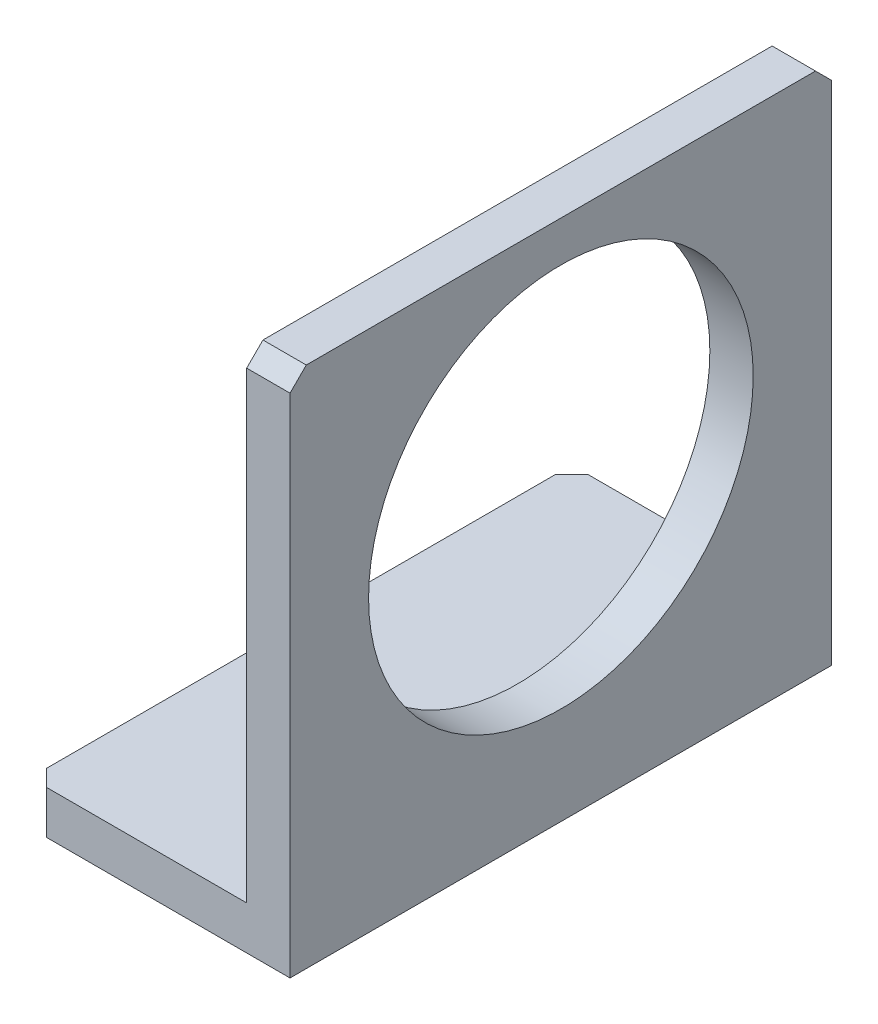
from build123d import *

# Parameters (mm, degrees)
EXTRUDE_1_DEPTH     = 50
CHAMFER_1_SIZE      = 3
CUT_EXTRUDE_1_REACH = 136.284
SKETCH_4_R          = 35.5


with BuildPart() as part:
    # 草图2 → 凸台-拉伸1 (new, symmetric)
    with BuildSketch(Plane(origin=(409.637600706, 0.5, -34.379468655), x_dir=(1, 0, 0), z_dir=(0, 0, 1))):
        Polygon((-409.637600706, 96), (-409.637600706, -0.5), (-457.637600706, -0.5), (-457.637600706, 7.5), (-417.637600706, 7.5), (-417.637600706, 96), align=None)
    extrude(amount=EXTRUDE_1_DEPTH, both=True)

    # 倒角1
    chamfer_1_edges = [part.edges().sort_by_distance(p)[0] for p in [
        (-48, 4, 15.620531345),
        (-4, 96.5, 15.620531345),
        (-48, 4, -84.379468655),
        (-4, 96.5, -84.379468655),
    ]]
    chamfer(chamfer_1_edges, length=CHAMFER_1_SIZE)

    # 草图4 → 切除-拉伸1 (cut, up to next)
    with BuildSketch(Plane.ZY.offset(8), mode=Mode.PRIVATE) as cut_extrude_1_sk1:
        with Locations((-34.379468655, 53.5)):
            Circle(SKETCH_4_R)
    cut_extrude_1_tool1 = extrude(cut_extrude_1_sk1.sketch, amount=-CUT_EXTRUDE_1_REACH, mode=Mode.PRIVATE) & part.part
    add(cut_extrude_1_tool1.solids().sort_by_distance((-8, 53.5, -34.379469))[0], mode=Mode.SUBTRACT)


solid = part.part
